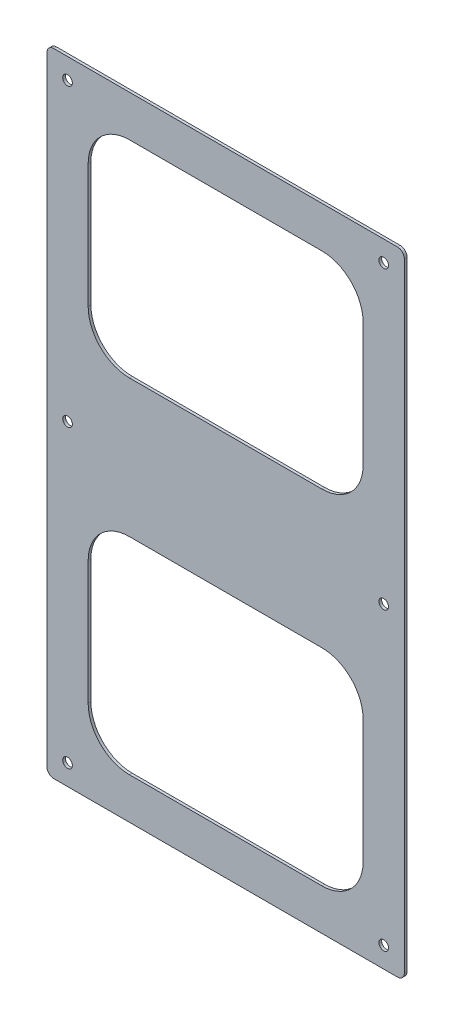
from build123d import *

# Parameters (mm, degrees)
SKETCH_1_W          = 260
SKETCH_1_H          = 460
EXTRUDE_1_DEPTH     = 2
FILLET_1_R          = 5
SKETCH_2_R          = 3.5
CUT_EXTRUDE_1_DEPTH = 529.397577587
CUT_EXTRUDE_2_DEPTH = 529.397577587


with BuildPart() as part:
    # 草图1 → 凸台-拉伸1 (new body)
    with BuildSketch(Plane.XY):
        with Locations((130, -230)):
            Rectangle(SKETCH_1_W, SKETCH_1_H)
    extrude(amount=EXTRUDE_1_DEPTH)

    # 圆角1
    fillet_1_edges = [part.edges().sort_by_distance(p)[0] for p in [
        (0, 0, 1),
        (260, 0, 1),
        (260, -460, 1),
        (0, -460, 1),
    ]]
    fillet(fillet_1_edges, radius=FILLET_1_R)

    # 草图2 → 切除-拉伸1 (cut, through all)
    with BuildSketch(Plane(origin=(0, 0, 0), x_dir=(-1, 0, 0), z_dir=(0, 0, -1))):
        with Locations((-245, -445)):
            Circle(SKETCH_2_R)
        with Locations((-15, -445)):
            Circle(SKETCH_2_R)
        with Locations((-245, -15)):
            Circle(SKETCH_2_R)
        with Locations((-15, -15)):
            Circle(SKETCH_2_R)
        with Locations((-245, -230)):
            Circle(SKETCH_2_R)
        with Locations((-15, -230)):
            Circle(SKETCH_2_R)
    extrude(amount=-CUT_EXTRUDE_1_DEPTH, mode=Mode.SUBTRACT)

    # 草图3 → 切除-拉伸2 (cut, through all)
    with BuildSketch(Plane(origin=(0, 0, 0), x_dir=(-1, 0, 0), z_dir=(0, 0, -1))):
        with BuildLine():
            Line((-60, -430), (-200, -430))
            ThreePointArc((-200, -430), (-221.213203436, -421.213203436), (-230, -400))
            Line((-230, -400), (-230, -310))
            ThreePointArc((-230, -310), (-221.213203436, -288.786796564), (-200, -280))
            Line((-200, -280), (-60, -280))
            ThreePointArc((-60, -280), (-38.786796564, -288.786796564), (-30, -310))
            Line((-30, -310), (-30, -400))
            ThreePointArc((-30, -400), (-38.786796564, -421.213203436), (-60, -430))
        make_face()
        with BuildLine():
            Line((-60, -180), (-200, -180))
            ThreePointArc((-200, -180), (-221.213203436, -171.213203436), (-230, -150))
            Line((-230, -150), (-230, -60))
            ThreePointArc((-230, -60), (-221.213203436, -38.786796564), (-200, -30))
            Line((-200, -30), (-60, -30))
            ThreePointArc((-60, -30), (-38.786796564, -38.786796564), (-30, -60))
            Line((-30, -60), (-30, -150))
            ThreePointArc((-30, -150), (-38.786796564, -171.213203436), (-60, -180))
        make_face()
    extrude(amount=-CUT_EXTRUDE_2_DEPTH, mode=Mode.SUBTRACT)


solid = part.part
